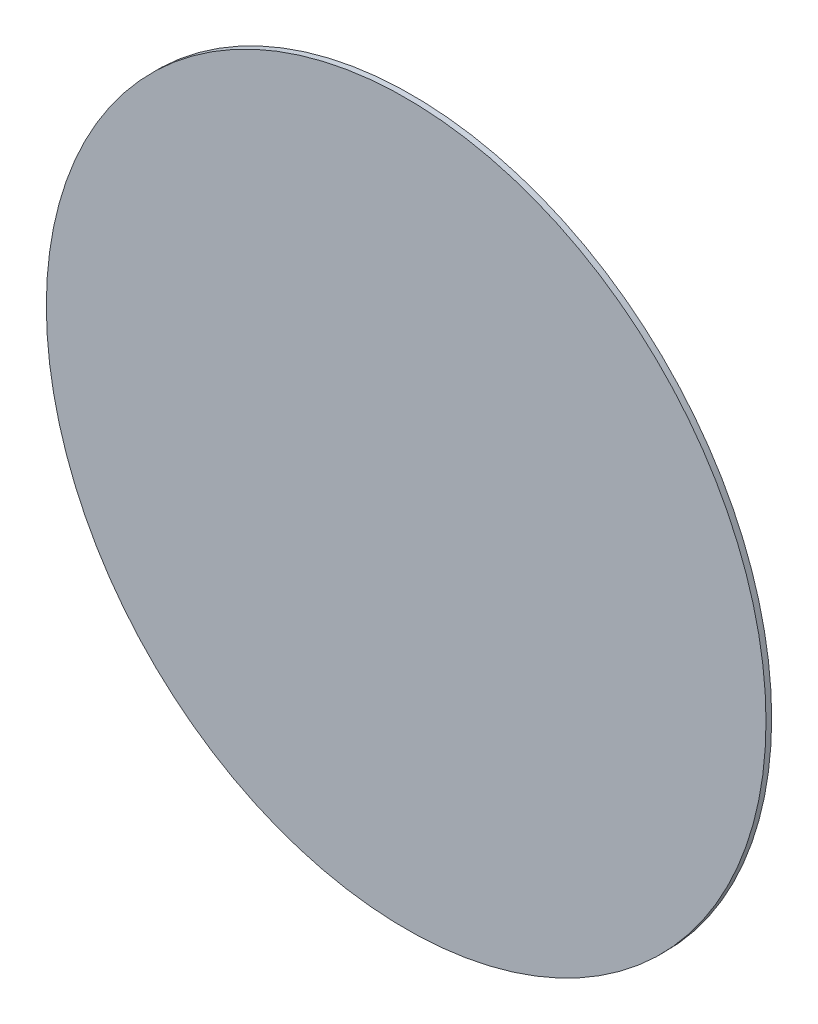
from build123d import *

# Parameters (mm, degrees)
SKETCH1_R           = 127
BOSS_EXTRUDE1_DEPTH = 2


with BuildPart() as part:
    # Sketch1 → Boss-Extrude1 (new body)
    with BuildSketch(Plane.XY):
        Circle(SKETCH1_R)
    extrude(amount=BOSS_EXTRUDE1_DEPTH)


solid = part.part
